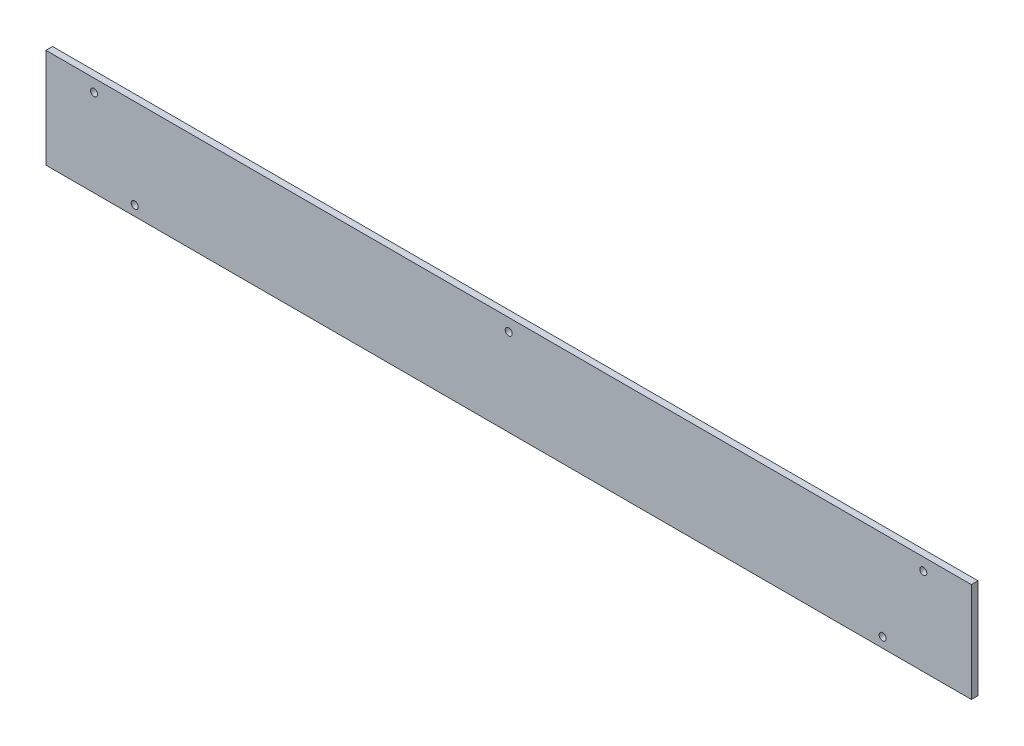
from build123d import *

# Parameters (mm, degrees)
SKETCH1_W              = 1116
SKETCH1_H              = 120
BOSS_EXTRUDE1_DEPTH    = 8
M10_TAPPED_HOLE1_D     = 8.5
M10_TAPPED_HOLE1_DEPTH = 24.5
M10_TAPPED_HOLE1_TIP   = 2.553657631


with BuildPart() as part:
    # Sketch1 → Boss-Extrude1 (new body)
    with BuildSketch(Plane.XY):
        Rectangle(SKETCH1_W, SKETCH1_H)
    extrude(amount=BOSS_EXTRUDE1_DEPTH)

    # M10 Tapped Hole1
    with Locations(Plane.XY.offset(8)):
        with Locations((-500, 45), (-451, -48), (0, 45), (500, 45), (451, -48)):
            Hole(M10_TAPPED_HOLE1_D / 2, depth=M10_TAPPED_HOLE1_DEPTH)
            with Locations((0, 0, -(M10_TAPPED_HOLE1_DEPTH + M10_TAPPED_HOLE1_TIP / 2))):  # 118° drill point
                Cone(0, M10_TAPPED_HOLE1_D / 2, M10_TAPPED_HOLE1_TIP, mode=Mode.SUBTRACT)


solid = part.part
